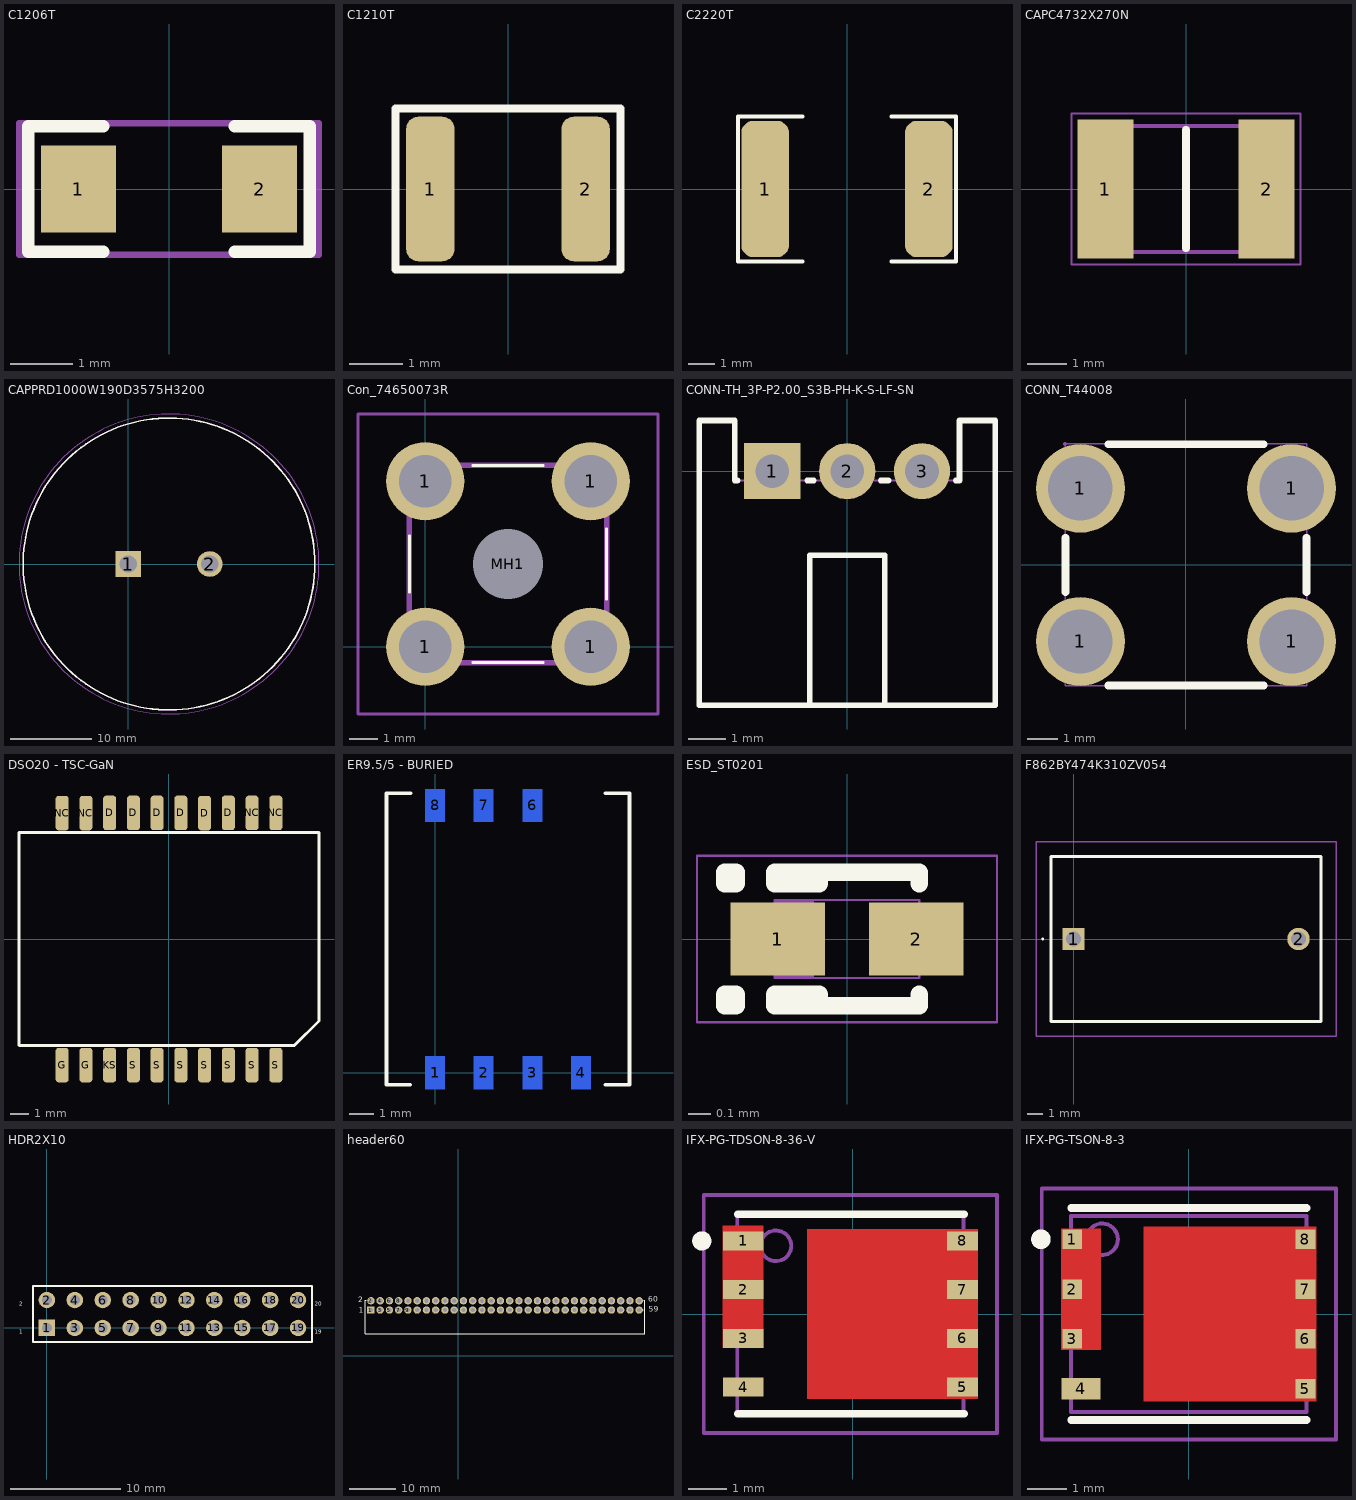
[diagram p0: the footprints below, top view; thin cyan lines are the x and y axes]
# Altium footprint library MISC82254-2.PcbLib: 93 footprints (part 2 of 6)
Each footprint in its own frame and in the unit in brackets; x right, y up, seen from the top. Pads: shape width x height; smd on the part's side, far side on the other; paste and mask are expansions set on the pad; w line width, h text height; cw(c..) or ccw(c..) is an arc to the next point about the centre after c.

## C1206T [mm]
pads (2):
  rect 1.2x1.4 smd: 1(-1.45,0) 2(1.45,0)
Top Overlay:
  lines w0.2: -1.051,-1 -2.25,-1 -2.25,1 -1.051,1 ; 1.051,-1 2.25,-1 2.25,1 1.051,1
Mechanical 15:
  lines w0.1: -2.4,-1.05 -2.4,1.05 2.4,1.05 2.4,-1.05 -2.4,-1.05
3D body "VJ1206A103JXATW1BC.stp": height 1.7, standoff 0, extent -1.6,-0.8 1.6,0.8

## C1210T [mm] "capacitor 1210 reflow soldering"
pads (2):
  rrect50% 0.9x2.7 smd: 1(-1.45,0) 2(1.45,0)
Top Overlay:
  lines w0.15: -2.1,-1.5 2.1,-1.5 2.1,1.5 -2.1,1.5 -2.1,-1.5
3D body "CAP1210.stp": height 0.92, standoff -0.02, extent -1.6,-1.25 1.6,1.25

## C2220T [mil]
height 110.24
pads (2):
  rrect50% 70x200 smd: 1(-120,0) 2(120,0)
Top Overlay:
  lines w5.91: -64.96,-106.3 -160,-106.3 -160,106.3 -64.96,106.3 ; 64.96,-106.3 160,-106.3 160,106.3 64.96,106.3
3D body: height 110.24, standoff 0, extent -120,-106.49 120,106.5

## CAPC4732X270N [mm]
pads (2):
  rect 1.43x3.52 smd: 1(-2.04,0) 2(2.04,0)
Top Overlay:
  lines w0.2: 0,-1.5 0,1.5
Mechanical 13:
  lines w0.1: -2.35,-1.6 -2.35,1.6 2.35,1.6 2.35,-1.6 -2.35,-1.6
Mechanical 15:
  lines w0.05: -2.905,-1.91 -2.905,1.91 2.905,1.91 2.905,-1.91 -2.905,-1.91
3D body "CKC18X153JDGACAUTO.stp": height 2.7, standoff 0, extent -2.55,-1.75 2.55,1.75

## CAPPRD1000W190D3575H3200 [mm]
pads (2):
  rect 3.15x3.15 hole 2.1: 1(0,0)
  round 3.15 hole 2.1: 2(10,0)
Top Overlay:
  circle w0.2: c5,0 r17.875
Mechanical 13:
  circle w0.1: c5,0 r17.875
Mechanical 15:
  circle w0.05: c5,0 r18.375
3D body "LGY1J472MELC30.stp": height 32, standoff -10, extent -13.25,-18.245 23.25,18.245

## Con_74650073R [mm]
pads (5):
  round 2.775 hole 1.85: 1(0,0) 1(0,5.87) 1(5.87,0) 1(5.87,5.87)
  round 1.25 hole 2.5 unplated: MH1(2.935,2.935)
Top Overlay:
  lines w0.1: -0.565,1.935 -0.565,3.935 -0.565,1.935 ; 1.685,-0.565 4.185,-0.565 1.685,-0.565 ; 1.685,6.435 4.185,6.435 1.685,6.435 ; 6.435,1.685 6.435,4.185 6.435,1.685
Mechanical 13:
  lines w0.2: -0.565,-0.565 -0.565,6.435 6.435,6.435 6.435,-0.565 -0.565,-0.565
Mechanical 15:
  lines w0.1: -2.388,-2.388 -2.388,8.258 8.258,8.258 8.258,-2.388 -2.388,-2.388
3D body "74650073R.stp": height 2.95, standoff -2.55, extent -0.65,-0.56 6.35,6.44

## CONN-TH_3P-P2.00_S3B-PH-K-S-LF-SN [mm]
pads (3):
  rect 1.5x1.5 hole 0.9: 1(-2,0)
  round 1.5 hole 0.9: 2(0,0) 3(2,0)
Top Overlay:
  lines w0.152: -2.93,-0.25 -3,-0.25 -3,1.35 -3.95,1.35 -3.95,-6.25 3.95,-6.25 3.95,1.35 3,1.35 3,-0.25 2.896,-0.25 ; -1.07,-0.25 -0.896,-0.25 ; -0.999,-6.25 -0.999,-2.25 1,-2.25 1,-6.25 ; 0.896,-0.25 1.104,-0.25
Mechanical 6:
  region: -4,-5.4 -4,-6.2 -3.9,-6.3 3.9,-6.3 4,-6.2 4,-5.6 3.9,-5.6 3.9,-6.2 -3.9,-6.2 -3.9,-5.4
Mechanical 15:
  region: -1.75,0.25 -1.75,-0.26 -2.25,-0.26 -2.25,0.24 -2.25,0.25
  region: 0.25,0.25 0.25,-0.26 -0.25,-0.26 -0.25,0.24 -0.25,0.25
  region: 2.25,0.25 2.25,-0.26 1.75,-0.26 1.75,0.24 1.75,0.25
  region: -2.25,0.25 -1.75,0.25 -1.75,-0.25 -2.25,-0.25
  region: -0.25,0.25 0.25,0.25 0.25,-0.25 -0.25,-0.25
  region: 1.75,0.25 2.25,0.25 2.25,-0.25 1.75,-0.25
  region: -3.89,-6.25 -3.89,-6.225 -3.925,-6.19 -3.975,-6.19 -4.01,-6.225 -4.01,-6.25 -4.01,-6.275 -3.975,-6.31 -3.925,-6.31 -3.89,-6.275
  lines w0.051: -3.95,-6.25 -3.95,1.35 -3,1.35 -3,-0.25 0,-0.25 3,-0.25 3,1.35 3.95,1.35 3.95,-6.25 -3.95,-6.25

## CONN_T44008 [mm]
pads (4):
  round 2.9 hole 2.1 paste-2539.97 mask+0.05: 1(-3.45,-2.5) 1(-3.45,2.5) 1(3.45,-2.5) 1(3.45,2.5)
Top Overlay:
  lines w0.254: -3.937,-0.889 -3.937,0.889 ; -2.54,-3.937 2.54,-3.937 ; -2.54,3.937 -1.778,3.937 2.54,3.937 ; 3.937,-0.889 3.937,0.889
Mechanical 15:
  region: -3.89,3.95 -3.891,3.974 -3.926,4.007 -3.974,4.007 -4.009,3.974 -4.01,3.95 -4.009,3.926 -3.974,3.893 -3.926,3.893 -3.891,3.926
  region: -3.95,1.75 -3.95,3.25 -2.95,3.25 -2.95,1.75
  region: 2.95,1.75 2.95,3.25 3.95,3.25 3.95,1.75
  region: 3.95,-1.75 3.95,-3.25 2.95,-3.25 2.95,-1.75
  region: -3.95,-3.25 -3.95,-1.75 -2.95,-1.75 -2.95,-3.25
  lines w0.051: -3.95,-3.95 -3.95,3.95 3.95,3.95 3.95,-3.95 -3.95,-3.95
3D body "3D_PCB1_2024-02-211.STEP": height 6.2, standoff -5, extent -3.951,-3.937 3.951,3.963

## DSO20 - TSC-GaN [mm]
height 3.5
pads (21):
  rrect50% 0.7x1.85 smd: D(-3.175,6.75) D(-1.905,6.75) D(-0.635,6.75) D(0.635,6.75) D(1.905,6.74) D(3.175,6.75) G(-5.715,-6.74) G(-4.445,-6.74) KS(-3.175,-6.74) NC(-5.715,6.74) NC(-4.445,6.74) NC(4.445,6.75) NC(5.715,6.75) S(-1.905,-6.74) S(-0.635,-6.74) S(0.635,-6.74) S(1.905,-6.74) S(3.175,-6.74) S(4.445,-6.74) S(5.715,-6.74)
  round 1 on Top Overlay: ""(7.363,-5.037)
Top Overlay:
  lines w0.15: -8.025,-5.675 -8.025,5.701 8.025,5.701 8.025,-4.375 6.701,-5.699 -8.001,-5.699 -8.025,-5.675
Top Paste:
  circle w0.013: c0,0 r0.1
3D body "PG-DSO-20-TSC.stp": height 3.5, standoff 0, extent -8.1,-7.1 8.1,7.1

## ER9.5/5 - BURIED [mm] "8 pin SM ER9.5/5 - Fits in PCB cutout with bottom side pads"
height 5.08
pads (8):
  rect 0.8x1.35 smd far side: 1(0,0) 2(2,0) 3(4,0) 4(6,0) 6(4,11) 7(2,11) 8(0,11)
  oval 0.8x1 on Top Overlay: ""(-1.3,0.1)
Top Overlay:
  lines w0.15: -1.02,-0.5 -2,-0.5 -2,11.5 -1,11.5 ; 7,-0.5 8,-0.5 8,11.5 7,11.5
3D body: height 2, standoff 1.5, extent -1,1 7,3
3D body: height 2, standoff 1.5, extent -1,8 7,10
3D body: height 3, standoff -3, extent -2,3 8,8
3D body: height -1.5, standoff -3, extent -1,1 7,3
3D body: height 2, standoff -2, extent -1,1.5 7,9.494
3D body: height -1.5, standoff -3, extent -1,8 7,10

## ESD_ST0201 [mm]
height 0.33
pads (2):
  rect 0.425x0.33 smd mask+0.05: 1(-0.312,0) 2(0.312,0)
Top Overlay:
  lines w0.08: -0.325,-0.275 -0.125,-0.275 ; -0.325,0.275 -0.125,0.275 ; -0.125,-0.3 -0.125,-0.25 -0.325,-0.25 -0.325,-0.3 0.325,-0.3 0.325,-0.25 ; -0.125,0.3 -0.125,0.25 -0.325,0.25 -0.325,0.3 0.325,0.3 0.325,0.25 ; -0.55,-0.3 -0.5,-0.3 -0.5,-0.25 -0.55,-0.25 -0.55,-0.3 ; -0.55,0.25 -0.55,0.3 -0.5,0.3 -0.5,0.25 -0.55,0.25
Mechanical 14:
  rectangle: -0.325,-0.175 -0.15,0.175
  lines w0.01: -0.325,-0.175 0.325,-0.175 0.325,0.175 -0.325,0.175 -0.325,-0.175
  text "'.Designator'" at 1.175,-2.025 h0.75
  text "K" at -0.575,-0.15 h0.45
Mechanical 16:
  lines w0.01: -0.675,-0.375 0.675,-0.375 0.675,0.375 -0.675,0.375 -0.675,-0.375
3D body "0201.STEP": height 0.34, standoff 0, extent -0.341,-0.165 0.339,0.165
3D body: height 0.33, standoff 0, extent -0.325,-0.175 0.325,0.175

## F862BY474K310ZV054 [mm]
pads (2):
  rect 1.5x1.5 hole 1: 1(0,0)
  round 1.5 hole 1: 2(15,0)
Top Overlay:
  lines w0.1: -2.1,0 ccw(c-2.05,0) -2,0 ccw(c-2.05,0) -2.1,0
  lines w0.2: -1.5,-5.5 -1.5,5.5 16.5,5.5 16.5,-5.5 -1.5,-5.5
Mechanical 13:
  lines w0.1: -1.5,-5.5 -1.5,5.5 16.5,5.5 16.5,-5.5 -1.5,-5.5
Mechanical 15:
  lines w0.1: -2.5,-6.5 -2.5,6.5 17.5,6.5 17.5,-6.5 -2.5,-6.5
3D body "F862BY474K310ZV054.stp": height 18, standoff -6.5, extent -1.25,-5.255 16.25,5.25

## HDR2X10 [mm] "Connector; Header; 10x2 Position"
pads (20):
  rect 1.5x1.5 hole 0.9: 1(0,0)
  round 1.5 hole 0.9: 2(0,2.54) 3(2.54,0) 4(2.54,2.54) 5(5.08,0) 6(5.08,2.54) 7(7.62,0) 8(7.62,2.54) 9(10.16,0) 10(10.16,2.54) 11(12.7,0) 12(12.7,2.54) 13(15.24,0) 14(15.24,2.54) 15(17.78,0) 16(17.78,2.54) 17(20.32,0) 18(20.32,2.54) 19(22.86,0) 20(22.86,2.54)
Top Overlay:
  lines w0.2: -1.27,-1.27 0.635,-1.27 24.13,-1.27 24.13,3.81 0.635,3.81 -1.27,3.81 -1.27,-1.27
  text "20" at 24.384,2.032 h0.38
  text "19" at 24.384,-0.508 h0.38
  text "1" at -2.54,-0.508 h0.38
  text "2" at -2.54,2.032 h0.38

## header60 [mm]
pads (60):
  rect 1.6x1.6 hole 0.914 paste-2539.97 mask+0.05: 1(-18.923,9.938)
  round 1.6 hole 0.914 paste-2539.97 mask+0.05: 2(-18.923,11.938) 3(-16.923,9.938) 4(-16.923,11.938) 5(-14.923,9.938) 6(-14.923,11.938) 7(-12.923,9.938) 8(-12.923,11.938) 9(-10.923,9.938) 10(-10.923,11.938) 11(-8.923,9.938) 12(-8.923,11.938) 13(-6.923,9.938) 14(-6.923,11.938) 15(-4.923,9.938) 16(-4.923,11.938) 17(-2.923,9.938) 18(-2.923,11.938) 19(-0.923,9.938) 20(-0.923,11.938) 21(1.077,9.938) 22(1.077,11.938) 23(3.077,9.938) 24(3.077,11.938) 25(5.077,9.938) 26(5.077,11.938) 27(7.077,9.938) 28(7.077,11.938) 29(9.077,9.938) 30(9.077,11.938) 31(11.077,9.938) 32(11.077,11.938) 33(13.077,9.938) 34(13.077,11.938) 35(15.077,9.938) 36(15.077,11.938) 37(17.077,9.938) 38(17.077,11.938) 39(19.077,9.938) 40(19.077,11.938) 41(21.077,9.938) 42(21.077,11.938) 43(23.077,9.938) 44(23.077,11.938) 45(25.077,9.938) 46(25.077,11.938) 47(27.077,9.938) 48(27.077,11.938) 49(29.077,9.938) 50(29.077,11.938) 51(31.077,9.938) 52(31.077,11.938) 53(33.077,9.938) 54(33.077,11.938) 55(35.077,9.938) 56(35.077,11.938) 57(37.077,9.938) 58(37.077,11.938) 59(39.077,9.938) 60(39.077,11.938)
Top Overlay:
  lines w0.254: -19.954,12.038 -20.173,12.038 -20.173,4.838 40.327,4.838 ; 40.058,10.054 40.292,10.054 ; 40.058,12.054 40.292,12.054 ; 40.336,4.838 40.336,12.038
  text "1" at -21.59,8.89 h2
  text "2" at -21.718,11.176 h2
  text "59" at 41.148,9.165 h2
  text "60" at 41.021,11.324 h2
3D body "3D_PCB1_2024-02-20new3.STEP": height 4.85, standoff -2.3, extent -20.116,4.752 40.39,12.044

## IFX-PG-TDSON-8-36-V [mm] "PG-TDSON-8-36, SMD, 1.27 mm pitch, 8 pin, 5.90 mm L X 5.15 mm W X 1.00 mm H body"
height 1
pads (8):
  rect 1.055x0.5 smd paste-0.527 mask+0: 1(-2.861,1.905)
  rect 1.055x0.5 smd paste-0.25 mask+0: 2(-2.861,0.635) 3(-2.861,-0.635) 4(-2.861,-1.905)
  rect 0.8x0.5 smd paste-0.4 mask+0: 5(2.862,-1.905) 6(2.862,-0.635) 7(2.862,0.635) 8(2.862,1.905)
Top Layer:
  region: -3.388,-0.885 -2.333,-0.885 -2.333,2.305 -3.388,2.305
  region: 3.262,2.205 -1.193,2.205 -1.193,-2.205 3.262,-2.205
Top Overlay:
  circle w0.25: c-3.939,1.905 r0.125
  lines w0.2: -3,-2.6 2.9,-2.6 ; -3,2.6 2.9,2.6
Top Paste:
  region: 2.411,-1.705 3.211,-1.705 3.211,-2.105 2.411,-2.105
  region: 2.411,-0.435 3.211,-0.435 3.211,-0.835 2.411,-0.835
  region: 2.411,0.835 3.211,0.835 3.211,0.435 2.411,0.435
  region: 2.411,2.105 3.211,2.105 3.211,1.705 2.411,1.705
  region: -0.944,-1.8 -0.944,-0.1 0.457,-0.1 0.457,-1.8
  region: 0.656,-1.8 0.656,-0.1 2.057,-0.1 2.057,-1.8
  region: 0.656,0.1 0.656,1.8 2.057,1.8 2.057,0.1
  region: -0.944,0.1 -0.944,1.8 0.457,1.8 0.457,0.1
  region: -3.339,-1.705 -2.539,-1.705 -2.539,-2.105 -3.339,-2.105
  region: -2.789,2.265 -2.388,2.265 -2.388,1.365 -2.789,1.365
  region: -2.789,1.165 -2.388,1.165 -2.388,0.265 -2.789,0.265
  region: -2.789,0.065 -2.388,0.065 -2.388,-0.835 -2.789,-0.835
  region: -3.338,2.105 -2.989,2.105 -2.989,1.705 -3.338,1.705
  region: -3.338,0.835 -2.989,0.835 -2.989,0.435 -3.338,0.435
  region: -3.338,-0.435 -2.989,-0.435 -2.989,-0.835 -3.338,-0.835
Top Solder:
  region: -2.838,2.305 -2.333,2.305 -2.333,-0.885 -2.838,-0.885
  region: -1.193,2.205 2.537,2.205 2.537,-2.205 -1.193,-2.205
Mechanical 3:
  text ".DESIGNATOR" at 0,0 h1.2
Mechanical 13:
  circle w0.1: c-2.006,1.778 r0.4
  lines w0.1: -3.013,-2.575 2.887,-2.575 2.887,2.575 -3.013,2.575 -3.013,-2.575
Mechanical 15:
  lines w0.1: -0.5,0 0.5,0 ; 0,-0.5 0,0.5 ; 3.761,-3.1 -3.889,-3.1 -3.889,3.1 3.761,3.1 ; 3.762,-3.1 3.762,3.1
3D body "PG-TDSON-8-36_Z8B00186404_V03_3D.stp": height 1.01, standoff 0, extent -3.174,-2.705 3.047,2.705

## IFX-PG-TSON-8-3 [mm] "Transistor; 1.27mm pitch, 8 pin, 6.00mm L X 5.00mm W X 1.1mm H body"
height 1.1
pads (8):
  rect 0.5x0.5 smd paste-0.5 mask-0.5: 1(-2.972,1.905) 2(-2.972,0.635) 3(-2.972,-0.635) 5(2.972,-1.905) 6(2.972,-0.635) 7(2.972,0.635) 8(2.972,1.905)
  rect 1x0.54 smd paste-1 mask+0: 4(-2.75,-1.905)
Top Layer:
  region: -3.25,2.175 -3.25,-0.905 -2.25,-0.905 -2.25,2.175
  region: 3.25,2.225 3.25,-2.225 -1.15,-2.225 -1.15,2.225
Top Overlay:
  circle w0.25: c-3.772,1.905 r0.125
  lines w0.2: -3,-2.7 3,-2.7 ; -3,2.7 3,2.7
Top Paste:
  region: -2.815,1.685 -3.205,1.685 -3.205,2.125 -2.815,2.125
  region: -2.815,0.415 -3.205,0.415 -3.205,0.855 -2.815,0.855
  region: -2.3,2.125 -2.3,1.275 -2.69,1.275 -2.69,2.125
  region: -2.3,1.065 -2.3,0.215 -2.69,0.215 -2.69,1.065
  region: -2.3,0 -2.3,-0.85 -2.69,-0.85 -2.69,0
  region: -2.815,-0.855 -3.205,-0.855 -3.205,-0.415 -2.815,-0.415
  region: 2.38,-0.415 2.38,-0.855 3.2,-0.855 3.2,-0.415
  region: 2.38,0.855 2.38,0.415 3.2,0.415 3.2,0.855
  region: 2.38,1.685 2.38,2.125 3.2,2.125 3.2,1.685
  region: -0.95,0.1 -0.95,1.6 0.55,1.6 0.55,0.1
  region: -0.95,-1.6 -0.95,-0.1 0.55,-0.1 0.55,-1.6
  region: 2.38,-2.125 2.38,-1.685 3.2,-1.685 3.2,-2.125
  region: 0.75,-1.6 0.75,-0.1 2.25,-0.1 2.25,-1.6
  region: 0.75,0.1 0.75,1.6 2.25,1.6 2.25,0.1
  region: -2.815,-2.125 -3.205,-2.125 -3.205,-1.685 -2.815,-1.685
  region: -2.3,-2.125 -2.69,-2.125 -2.69,-1.685 -2.299,-1.685
Top Solder:
  region: 3.25,2.175 3.25,1.635 2.53,1.635 2.53,0.905 3.25,0.905 3.25,0.365 2.53,0.365 2.53,-0.365 3.25,-0.365 3.25,-0.905 2.53,-0.905 2.53,-1.635 3.25,-1.635 3.25,-2.175 2.52,-2.175 2.52,-2.225 -1.15,-2.225 -1.15,2.225 2.52,2.225 2.52,2.175
  region: -3.25,2.175 -2.25,2.175 -2.25,-0.905 -3.25,-0.905 -3.25,-0.365 -2.8,-0.365 -2.8,0.365 -3.25,0.365 -3.25,0.905 -2.8,0.905 -2.8,1.635 -3.25,1.635
Mechanical 3:
  text ".DESIGNATOR" at 0,0 h1.2
Mechanical 13:
  circle w0.1: c-2.21,1.905 r0.4
  lines w0.1: -3,-2.5 3,-2.5 3,2.5 -3,2.5 -3,-2.5
Mechanical 15:
  lines w0.1: -0.5,0 0.5,0 ; 0,-0.5 0,0.5 ; -3.75,-3.2 -3.75,3.2 3.75,3.2 3.75,-3.2 -3.75,-3.2
3D body "BSC027N10NS5.STEP": height 1.1, standoff 0, extent -3,-2.5 3,2.5